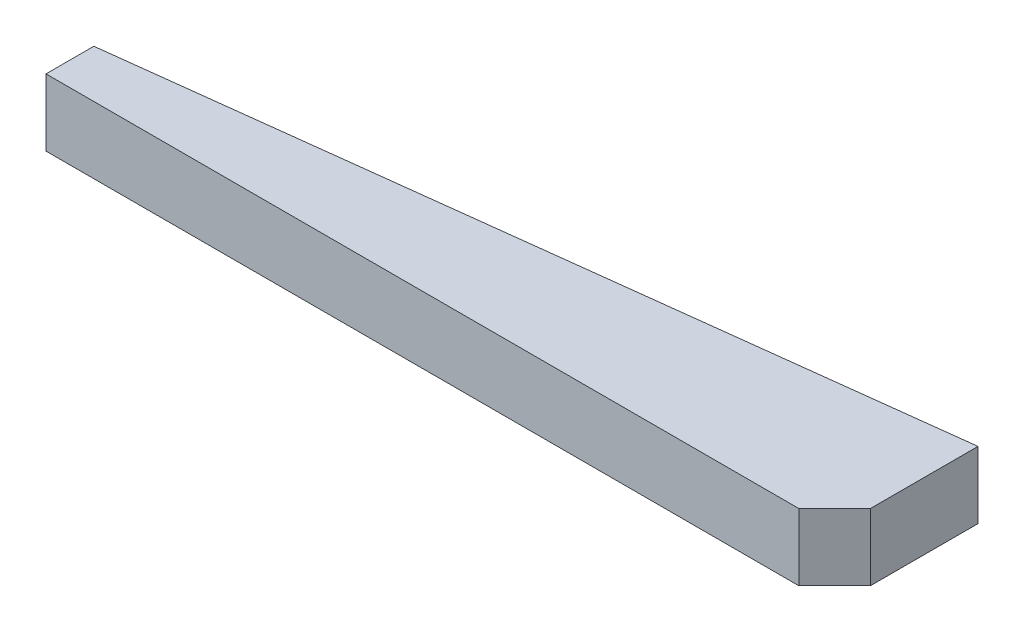
from build123d import *

# Parameters (mm, degrees)
BOSS_EXTRUDE1_DEPTH = 28


with BuildPart() as part:
    # Sketch1 → Boss-Extrude1 (new body)
    with BuildSketch(Plane(origin=(0, 0, 0), x_dir=(1, 0, 0), z_dir=(0, 1, 0))):
        Polygon((2750.872583656, 1604.162796977), (3065.872583656, 1604.162796977), (3080.872583656, 1619.162796977), (3080.872583656, 1664.162796977), (2750.872583656, 1624.162796977), align=None)
    extrude(amount=BOSS_EXTRUDE1_DEPTH)


solid = part.part
